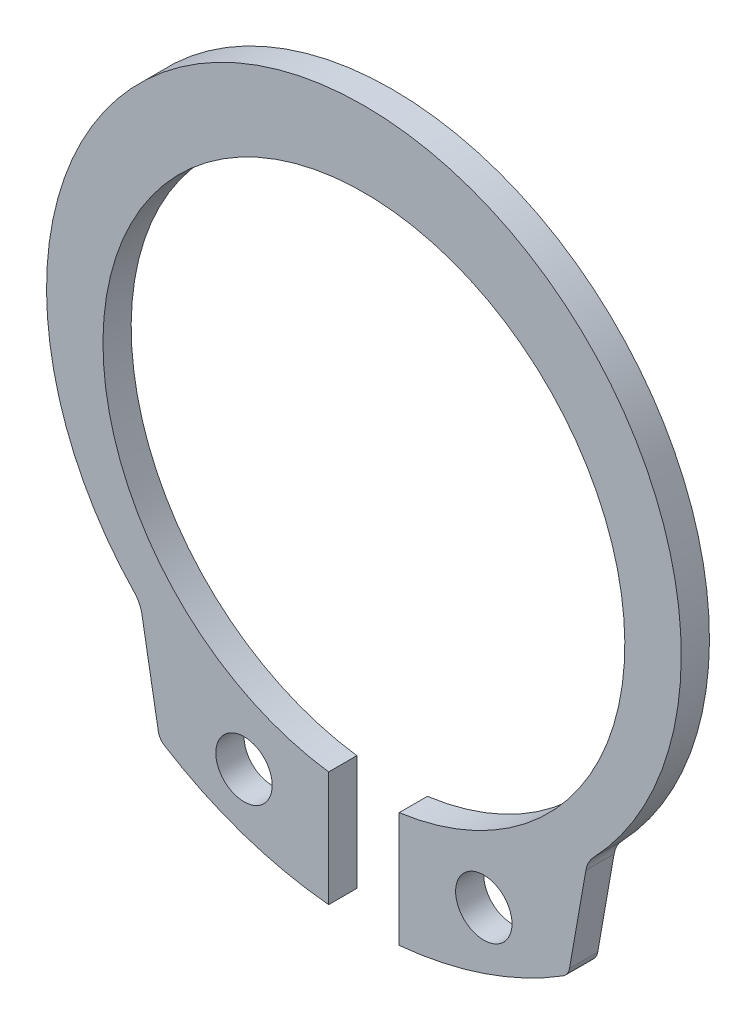
SolidWorks part; units mm, degrees
ref_plane "前视基准面" through (0, 0, 0) normal (0, 0, 1) x (1, 0, 0)
ref_plane "上视基准面" through (0, 0, 0) normal (0, 1, 0) x (1, 0, 0)
ref_plane "右视基准面" through (0, 0, 0) normal (1, 0, 0) x (0, 0, -1)
other "Configuration Table"
sketch "草图1" plane through (0, 0, 0) normal (0, 0, 1) x (1, 0, 0)
  line L7 (-14.5762, -23.2075) -> (-15.7425, -16.5805)
  line L8 (14.5762, -23.2075) -> (15.7425, -16.5805)
  line L9 (-2.5, -27.8223) -> (-2.5, -19.6703)
  line L10 (2.5, -27.8223) -> (2.5, -19.6703)
  arc A0 (16.2663, -15.5453) -> (-16.2663, -15.5453) centre (0, 0) ccw
  arc A1 (2.5, -19.6703) -> (-2.5, -19.6703) centre (0, -1.34) ccw
  arc A2 (-14.1222, -23.8816) -> (-2.5, -27.8223) centre (0, -1.34) ccw
  arc A3 (2.5, -27.8223) -> (14.1222, -23.8816) centre (0, -1.34) ccw
  circle A4 centre (-8.5, -22.5) radius 2
  circle A5 centre (8.5, -22.5) radius 2
  arc A6 (-15.7425, -16.5805) -> (-16.2663, -15.5453) centre (-17.7122, -16.9271) ccw
  arc A7 (15.7425, -16.5805) -> (16.2663, -15.5453) centre (17.7122, -16.9271) cw
  arc A8 (-14.1222, -23.8816) -> (-14.5762, -23.2075) centre (-13.5913, -23.0341) cw
  arc A9 (14.5762, -23.2075) -> (14.1222, -23.8816) centre (13.5913, -23.0341) cw
  point P10 (0, -44.6136)
  point P12 (0, -27.94)
  point P14 (0, -44.6136)
  point P16 (0, -44.6136)
  point P22 (0, -32.2007)
  point P28 (0, -22.5)
  dimension "D1" = 45
  dimension "D3" = 37
  dimension "D6" = 4
  dimension "D7" = 4
  dimension "D8" = 2
  dimension "D9" = 2
  dimension "D10" = 1
  dimension "D11" = 1
  dimension "D2" = 1.34
extrude "凸台-拉伸1" add sketch "草图1" along normal blind 2
